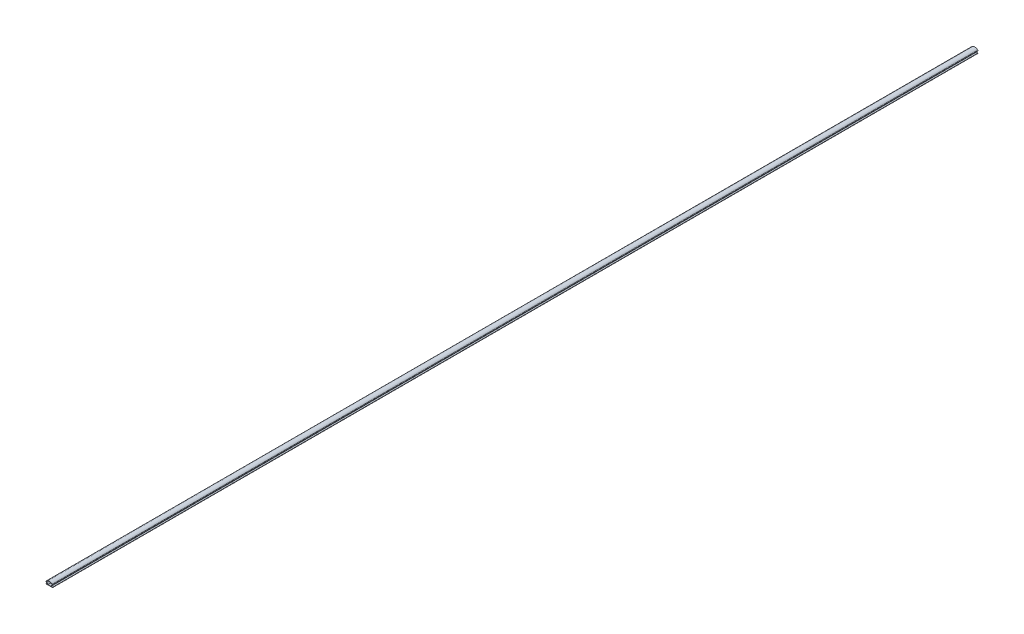
from build123d import *

# Parameters (mm, degrees)
EXTRUDE_1_DEPTH = 705


with BuildPart() as part:
    # 草图1 → 凸台-拉伸1 (new, symmetric)
    with BuildSketch(Plane.XY):
        with BuildLine():
            Line((-4.556913863, 4.138102128), (-2.645672962, 1.79891143))
            Line((-2.645672962, 1.79891143), (-5, 1.79891143))
            Line((-5, 1.79891143), (-5, 1.29891143))
            Line((-5, 1.29891143), (1.591473901, 1.29891143))
            Line((1.591473901, 1.29891143), (5, 1.29891143))
            Line((5, 1.29891143), (5, 1.79891143))
            Line((5, 1.79891143), (2.645672962, 1.79891143))
            Line((2.645672962, 1.79891143), (4.556913863, 4.138102128))
            ThreePointArc((4.556913863, 4.138102128), (4.780792009, 4.829714088), (4.47713902, 5.490201325))
            ThreePointArc((4.47713902, 5.490201325), (0, 7.29891143), (-4.47713902, 5.490201325))
            ThreePointArc((-4.47713902, 5.490201325), (-4.780792009, 4.829714088), (-4.556913863, 4.138102128))
        make_face()
        with BuildLine():
            Line((-2, 1.79891143), (2, 1.79891143))
            Line((2, 1.79891143), (4.169720942, 4.454458955))
            ThreePointArc((4.169720942, 4.454458955), (4.281660015, 4.800264935), (4.12983352, 5.130508554))
            ThreePointArc((4.12983352, 5.130508554), (0, 6.79891143), (-4.12983352, 5.130508554))
            ThreePointArc((-4.12983352, 5.130508554), (-4.281660015, 4.800264935), (-4.169720942, 4.454458955))
            Line((-4.169720942, 4.454458955), (-2, 1.79891143))
        make_face(mode=Mode.SUBTRACT)
    extrude(amount=EXTRUDE_1_DEPTH, both=True)


solid = part.part
